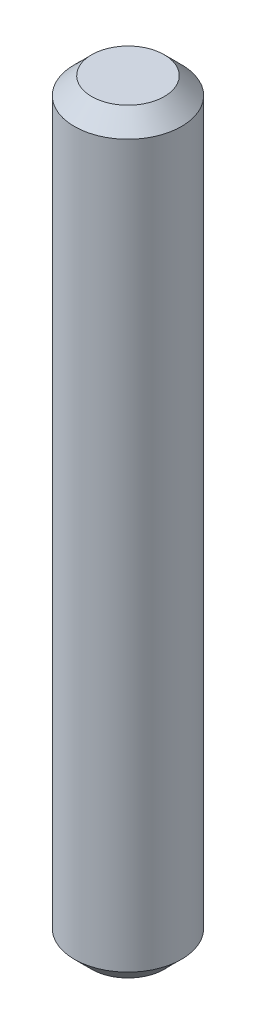
from build123d import *

# Parameters (mm, degrees)
SKETCH1_R           = 0.7874
BOSS_EXTRUDE1_DEPTH = 11.1125
CHAMFER1_SIZE       = 0.254


with BuildPart() as part:
    # Sketch1 → Boss-Extrude1 (new body)
    with BuildSketch(Plane(origin=(0, 0, 0), x_dir=(1, 0, 0), z_dir=(0, 1, 0))):
        with Locations(Location((0, 0, 0), (0, 0, 270))):
            Circle(SKETCH1_R)
    extrude(amount=BOSS_EXTRUDE1_DEPTH)

    # Chamfer1
    chamfer1_edges = [part.edges().sort_by_distance(p)[0] for p in [
        (0, 0, -0.7874),
        (0, 11.1125, -0.7874),
    ]]
    chamfer(chamfer1_edges, length=CHAMFER1_SIZE)


solid = part.part
